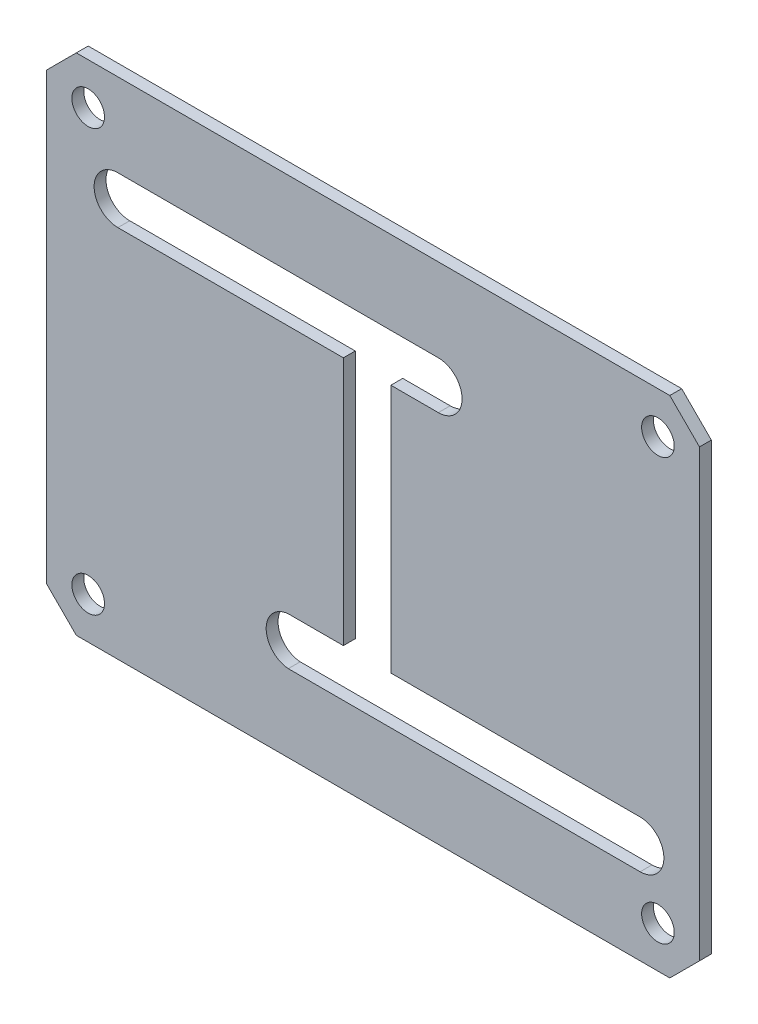
from build123d import *

# Parameters (mm, degrees)
EXTRUDE_1_DEPTH     = 2
CUT_EXTRUDE_1_DEPTH = 2
SKETCH_3_R          = 2.75
CUT_EXTRUDE_2_DEPTH = 2


with BuildPart() as part:
    # 草图1 → 凸台-拉伸1 (new body)
    with BuildSketch(Plane.XY):
        Polygon((357, 44.4274829), (457, 44.4274829), (462, 49.4274829), (462, 124.4274829), (457, 129.4274829), (357, 129.4274829), (352, 124.4274829), (352, 49.4274829), align=None)
    extrude(amount=EXTRUDE_1_DEPTH)

    # 草图2 → 切除-拉伸1 (cut)
    with BuildSketch(Plane.XY.offset(2)):
        with BuildLine():
            Line((452, 57.4274829), (392.718534883, 57.4274829))
            ThreePointArc((392.718534883, 57.4274829), (389, 61.708948017), (393.281465117, 65.4274829))
            Line((393.281465117, 65.4274829), (402, 65.4274829))
            Line((402, 65.4274829), (402, 107.4274829))
            Line((402, 107.4274829), (364, 107.4274829))
            ThreePointArc((364, 107.4274829), (360, 111.4274829), (364, 115.4274829))
            Line((364, 115.4274829), (418, 115.4274829))
            ThreePointArc((418, 115.4274829), (422, 111.4274829), (418, 107.4274829))
            Line((418, 107.4274829), (410, 107.4274829))
            Line((410, 107.4274829), (410, 65.4274829))
            Line((410, 65.4274829), (452, 65.4274829))
            ThreePointArc((452, 65.4274829), (456, 61.4274829), (452, 57.4274829))
        make_face()
    extrude(amount=-CUT_EXTRUDE_1_DEPTH, mode=Mode.SUBTRACT)

    # 草图3 → 切除-拉伸2 (cut)
    with BuildSketch(Plane.XY.offset(2)):
        with Locations((455, 51.4274829)):
            Circle(SKETCH_3_R)
        with Locations((359, 51.4274829)):
            Circle(SKETCH_3_R)
        with Locations((455, 122.4274829)):
            Circle(SKETCH_3_R)
        with Locations((359, 122.4274829)):
            Circle(SKETCH_3_R)
    extrude(amount=-CUT_EXTRUDE_2_DEPTH, mode=Mode.SUBTRACT)


solid = part.part
